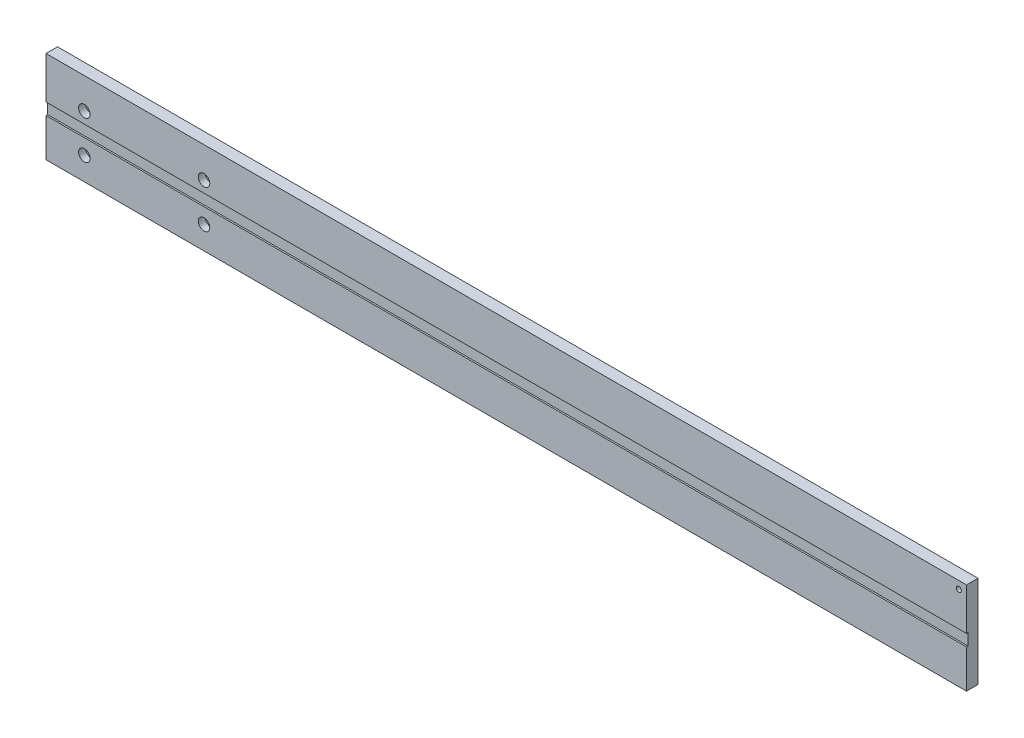
from build123d import *

# Parameters (mm, degrees)
SKETCH_1_W                  = 1200
SKETCH_1_H                  = 120
EXTRUDE_1_DEPTH             = 7.5
HOLE_WIZARD_3_D             = 6.6
HOLE_WIZARD_3_CBORE_D       = 11
HOLE_WIZARD_3_CBORE_DEPTH   = 6.8
HOLE_WIZARD_3_2_D           = 9
HOLE_WIZARD_3_2_CBORE_D     = 15
HOLE_WIZARD_3_2_CBORE_DEPTH = 9
SKETCH_7_W                  = 2
SKETCH_7_H                  = 15.2
CUT_EXTRUDE_1_DEPTH         = 1202.5224717


with BuildPart() as part:
    # 草图1 → 凸台-拉伸1 (new, symmetric)
    with BuildSketch(Plane.XY):
        Rectangle(SKETCH_1_W, SKETCH_1_H)
    extrude(amount=EXTRUDE_1_DEPTH, both=True)

    # Hole Wizard 3 (through all)
    with Locations(Plane(origin=(590, 50, -7.5), x_dir=(-1, 0, 0), z_dir=(0, 0, -1))):
        with Locations((0, 0)):
            CounterBoreHole(HOLE_WIZARD_3_D / 2, HOLE_WIZARD_3_CBORE_D / 2, HOLE_WIZARD_3_CBORE_DEPTH)

    # Hole Wizard 3 2 (through all)
    with Locations(Plane(origin=(-550, 20, 7.5), x_dir=(1, 0, 0), z_dir=(0, 0, 1))):
        with Locations((0, 0), (156, 0), (156, -50), (0, -50)):
            CounterBoreHole(HOLE_WIZARD_3_2_D / 2, HOLE_WIZARD_3_2_CBORE_D / 2, HOLE_WIZARD_3_2_CBORE_DEPTH)

    # 草图7 → 切除-拉伸1 (cut, through all)
    with BuildSketch(Plane(origin=(600, 0, 0), x_dir=(0, 0, -1), z_dir=(1, 0, 0))):
        with Locations((-6.5, -2.4)):
            Rectangle(SKETCH_7_W, SKETCH_7_H)
    extrude(amount=-CUT_EXTRUDE_1_DEPTH, mode=Mode.SUBTRACT)


solid = part.part
